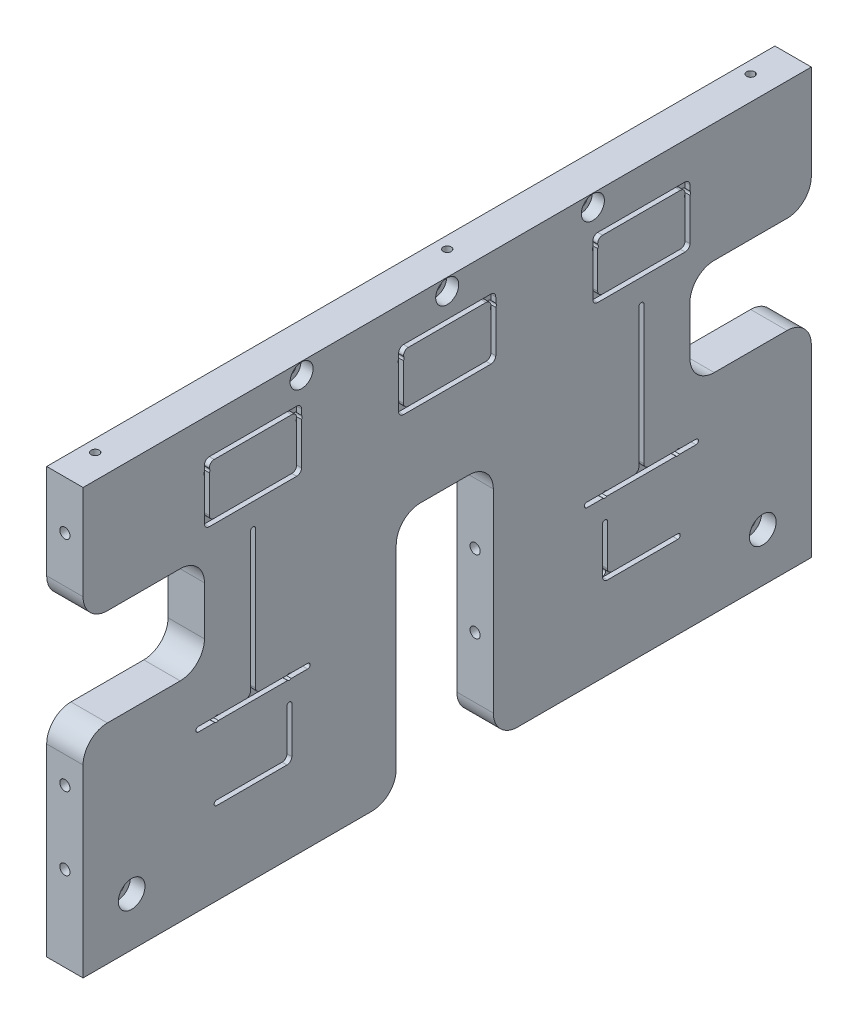
from build123d import *

# Parameters (mm, degrees)
SKETCH_2_W                                         = 300
SKETCH_2_H                                         = 175
BOSS_EXTRUDE_1_DEPTH                               = 15
SKETCH_7_W                                         = 15
SKETCH_7_H                                         = 40
CUT_EXTRUDE_1_DEPTH                                = 100
FILLET_1_R                                         = 10
SKETCH_8_W                                         = 15
SKETCH_8_H                                         = 40
CUT_EXTRUDE_2_DEPTH                                = 50
FILLET_2_R                                         = 10
SKETCH_9_R                                         = 2
CUT_EXTRUDE_3_DEPTH                                = 313.859792879
SKETCH_10_R                                        = 2
CUT_EXTRUDE_4_DEPTH                                = 313.859792879
LINEAR_PATTERN_1_COUNT                             = 2
LINEAR_PATTERN_1_PITCH                             = 30
M5_TAPPED_HOLE_1_AT_2_COUNT                        = 2
M5_TAPPED_HOLE_1_AT_2_PITCH                        = 90
M5_TAPPED_HOLE_1_AT_3_COUNT                        = 2
M5_TAPPED_HOLE_1_AT_3_PITCH                        = 120
M5_SOCKET_HEAD_CAP_SCREW_COUNTERBORE_1_D           = 5.5
M5_SOCKET_HEAD_CAP_SCREW_COUNTERBORE_1_CBORE_D     = 9.5
M5_SOCKET_HEAD_CAP_SCREW_COUNTERBORE_1_CBORE_DEPTH = 5
LINEAR_PATTERN_2_COUNT                             = 3
LINEAR_PATTERN_2_PITCH                             = 60
M6_SOCKET_HEAD_CAP_SCREW_COUNTERBORE_1_D           = 6.6
M6_SOCKET_HEAD_CAP_SCREW_COUNTERBORE_1_CBORE_D     = 11
M6_SOCKET_HEAD_CAP_SCREW_COUNTERBORE_1_CBORE_DEPTH = 6
CUT_EXTRUDE_5_DEPTH                                = 2
M5_TAPPED_HOLE_2_D                                 = 4.2
M5_TAPPED_HOLE_2_DEPTH                             = 12.4
M5_TAPPED_HOLE_2_TIP                               = 1.2618073
LINEAR_PATTERN_3_COUNT                             = 2
LINEAR_PATTERN_3_PITCH                             = 38
CUT_EXTRUDE_6_DEPTH                                = 2
LINEAR_PATTERN_4_COUNT                             = 2
LINEAR_PATTERN_4_PITCH                             = 30
LINEAR_PATTERN_5_COUNT                             = 2
LINEAR_PATTERN_5_PITCH                             = 80
LINEAR_PATTERN_6_COUNT                             = 2
LINEAR_PATTERN_6_PITCH                             = 80
CUT_EXTRUDE_7_DEPTH                                = 2
M4_TAPPED_HOLE_2_D                                 = 3.3
M4_TAPPED_HOLE_2_DEPTH                             = 10.1
M4_TAPPED_HOLE_2_TIP                               = 0.991420021
M5_TAPPED_HOLE_3_D                                 = 4.2
M5_TAPPED_HOLE_3_DEPTH                             = 12.4
M5_TAPPED_HOLE_3_TIP                               = 1.2618073


with BuildPart() as part:
    # Sketch 2 → Boss-Extrude 1 (new body)
    with BuildSketch(Plane(origin=(0, 0, 0), x_dir=(0, 0, -1), z_dir=(1, 0, 0))):
        Rectangle(SKETCH_2_W, SKETCH_2_H)
    extrude(amount=BOSS_EXTRUDE_1_DEPTH)

    # Sketch 3 → M4 Tapped Hole 1 (revolve, cut)
    with BuildSketch(Plane(origin=(5, 87.5, -135), x_dir=(0, 0, 1), z_dir=(1, 0, 0))):
        Polygon((0, 0), (0, 11.091420021), (1.65, 10.1), (1.65, 0), align=None)
    m4_tapped_hole_1 = revolve(axis=Axis((5, 93.85, -135), (0, -1, 0)), mode=Mode.SUBTRACT)

    # Mirror 1: M4 Tapped Hole 1 across plane
    add(m4_tapped_hole_1.mirror(Plane.XY), mode=Mode.SUBTRACT)

    # Sketch 7 → Cut-Extrude 1 (cut)
    with BuildSketch(Plane.XZ.offset(87.5)):
        with Locations((7.5, 1)):
            Rectangle(SKETCH_7_W, SKETCH_7_H)
    extrude(amount=-CUT_EXTRUDE_1_DEPTH, mode=Mode.SUBTRACT)

    # Fillet 1
    fillet_1_edges = [part.edges().sort_by_distance(p)[0] for p in [
        (7.5, 12.5, 21),
        (7.5, 12.5, -19),
        (7.5, -87.5, -19),
        (7.5, -87.5, 21),
    ]]
    fillet(fillet_1_edges, radius=FILLET_1_R)

    # Sketch 8 → Cut-Extrude 2 (cut)
    with BuildSketch(Plane(origin=(0, 0, -150), x_dir=(-1, 0, 0), z_dir=(0, 0, -1))):
        with Locations((-7.5, 18.5)):
            Rectangle(SKETCH_8_W, SKETCH_8_H)
    cut_extrude_2 = extrude(amount=-CUT_EXTRUDE_2_DEPTH, mode=Mode.SUBTRACT)

    # Mirror 2: Cut-Extrude 2 across plane
    add(cut_extrude_2.mirror(Plane.XY), mode=Mode.SUBTRACT)

    # Fillet 2
    fillet_2_edges = [part.edges().sort_by_distance(p)[0] for p in [
        (7.5, -1.5, -100),
        (7.5, 38.5, -100),
        (7.5, 38.5, -150),
        (7.5, -1.5, -150),
        (7.5, 38.5, 150),
        (7.5, -1.5, 150),
        (7.5, 38.5, 100),
        (7.5, -1.5, 100),
    ]]
    fillet(fillet_2_edges, radius=FILLET_2_R)

    # Sketch 9 → Cut-Extrude 3 (cut, through all)
    with BuildSketch(Plane.XY.offset(150)):
        with Locations((7.5, 67.5)):
            Circle(SKETCH_9_R)
    extrude(amount=-CUT_EXTRUDE_3_DEPTH, mode=Mode.SUBTRACT)

    # Sketch 10 → Cut-Extrude 4 (cut, through all)
    with BuildSketch(Plane.XY.offset(150)):
        with Locations((7.5, -22.5)):
            Circle(SKETCH_10_R)
    cut_extrude_4 = extrude(amount=-CUT_EXTRUDE_4_DEPTH, mode=Mode.SUBTRACT)

    # Linear Pattern 1: Cut-Extrude 4 ×2
    with Locations(*[(0, -i * LINEAR_PATTERN_1_PITCH, 0) for i in range(1, LINEAR_PATTERN_1_COUNT)]):
        add(cut_extrude_4, mode=Mode.SUBTRACT)

    # Sketch 11 → M5 Tapped Hole 1 (revolve, cut)
    with BuildSketch(Plane(origin=(7.5, 67.5, 150), x_dir=(0, -1, 0), z_dir=(1, 0, 0))):
        Polygon((0, 0), (0, 13.6618073), (2.1, 12.4), (2.1, 0), align=None)
    m5_tapped_hole_1 = revolve(axis=Axis((7.5, 67.5, 156.35), (0, 0, -1)), mode=Mode.SUBTRACT)

    # M5 Tapped Hole 1 at 2: M5 Tapped Hole 1 ×2
    with Locations(*[(0, -i * M5_TAPPED_HOLE_1_AT_2_PITCH, 0) for i in range(1, M5_TAPPED_HOLE_1_AT_2_COUNT)]):
        add(m5_tapped_hole_1, mode=Mode.SUBTRACT)

    # M5 Tapped Hole 1 at 3: M5 Tapped Hole 1 ×2
    with Locations(*[(0, -i * M5_TAPPED_HOLE_1_AT_3_PITCH, 0) for i in range(1, M5_TAPPED_HOLE_1_AT_3_COUNT)]):
        add(m5_tapped_hole_1, mode=Mode.SUBTRACT)

    # Mirror 4: M5 Tapped Hole 1 across plane
    add(m5_tapped_hole_1.mirror(Plane.XY), mode=Mode.SUBTRACT)

    # Mirror 4 copy 1 sketch → Mirror 4 copy 1 (revolve, cut)
    with BuildSketch(Plane(origin=(7.5, -22.5, -150), x_dir=(0, -1, 0), z_dir=(1, 0, 0))):
        Polygon((0, 0), (0, -13.6618073), (2.1, -12.4), (2.1, 0), align=None)
    revolve(axis=Axis((7.5, -22.5, -156.35), (0, 0, -1)), mode=Mode.SUBTRACT)

    # Mirror 4 copy 2 sketch → Mirror 4 copy 2 (revolve, cut)
    with BuildSketch(Plane(origin=(7.5, -52.5, -150), x_dir=(0, -1, 0), z_dir=(1, 0, 0))):
        Polygon((0, 0), (0, -13.6618073), (2.1, -12.4), (2.1, 0), align=None)
    revolve(axis=Axis((7.5, -52.5, -156.35), (0, 0, -1)), mode=Mode.SUBTRACT)

    # M5 Socket Head Cap Screw Counterbore 1 (through all)
    with Locations(Plane(origin=(15, 0, 0), x_dir=(0, 0, -1), z_dir=(1, 0, 0))):
        with Locations((-60, 82.5)):
            m5_socket_head_cap_screw_counterbore_1 = CounterBoreHole(M5_SOCKET_HEAD_CAP_SCREW_COUNTERBORE_1_D / 2, M5_SOCKET_HEAD_CAP_SCREW_COUNTERBORE_1_CBORE_D / 2, M5_SOCKET_HEAD_CAP_SCREW_COUNTERBORE_1_CBORE_DEPTH)

    # Linear Pattern 2: M5 Socket Head Cap Screw Counterbore 1 ×3
    with Locations(*[(0, 0, -i * LINEAR_PATTERN_2_PITCH) for i in range(1, LINEAR_PATTERN_2_COUNT)]):
        add(m5_socket_head_cap_screw_counterbore_1, mode=Mode.SUBTRACT)

    # M6 Socket Head Cap Screw Counterbore 1 (through all)
    with Locations(Plane(origin=(15, 0, 0), x_dir=(0, 0, -1), z_dir=(1, 0, 0))):
        with Locations((-130, -67.5)):
            m6_socket_head_cap_screw_counterbore_1 = CounterBoreHole(M6_SOCKET_HEAD_CAP_SCREW_COUNTERBORE_1_D / 2, M6_SOCKET_HEAD_CAP_SCREW_COUNTERBORE_1_CBORE_D / 2, M6_SOCKET_HEAD_CAP_SCREW_COUNTERBORE_1_CBORE_DEPTH)

    # Mirror 5: M6 Socket Head Cap Screw Counterbore 1 across plane
    add(m6_socket_head_cap_screw_counterbore_1.mirror(Plane.XY), mode=Mode.SUBTRACT)

    # Sketch 18 → Cut-Extrude 5 (cut)
    with BuildSketch(Plane(origin=(15, 0, 0), x_dir=(0, 0, -1), z_dir=(1, 0, 0))):
        with BuildLine():
            Line((-98, 72.5), (-62, 72.5))
            ThreePointArc((-62, 72.5), (-60.585786438, 71.914213562), (-60, 70.5))
            Line((-60, 70.5), (-60, 49.5))
            ThreePointArc((-60, 49.5), (-60.585786438, 48.085786438), (-62, 47.5))
            Line((-62, 47.5), (-98, 47.5))
            ThreePointArc((-98, 47.5), (-99.414213562, 48.085786438), (-100, 49.5))
            Line((-100, 49.5), (-100, 70.5))
            ThreePointArc((-100, 70.5), (-99.414213562, 71.914213562), (-98, 72.5))
        make_face()
        with BuildLine():
            Line((-96, 70.5), (-64, 70.5))
            ThreePointArc((-64, 70.5), (-62.585786438, 69.914213562), (-62, 68.5))
            Line((-62, 68.5), (-62, 51.5))
            ThreePointArc((-62, 51.5), (-62.585786438, 50.085786438), (-64, 49.5))
            Line((-64, 49.5), (-96, 49.5))
            ThreePointArc((-96, 49.5), (-97.414213562, 50.085786438), (-98, 51.5))
            Line((-98, 51.5), (-98, 68.5))
            ThreePointArc((-98, 68.5), (-97.414213562, 69.914213562), (-96, 70.5))
        make_face(mode=Mode.SUBTRACT)
    cut_extrude_5 = extrude(amount=-CUT_EXTRUDE_5_DEPTH, mode=Mode.SUBTRACT)

    # M5 Tapped Hole 2
    with Locations(Plane(origin=(0, 0, 21), x_dir=(-1, 0, 0), z_dir=(0, 0, -1))):
        with Locations((-7.5, -22.5), (-7.5, -52.5)):
            Hole(M5_TAPPED_HOLE_2_D / 2, depth=M5_TAPPED_HOLE_2_DEPTH)
            with Locations((0, 0, -(M5_TAPPED_HOLE_2_DEPTH + M5_TAPPED_HOLE_2_TIP / 2))):  # 118° drill point
                Cone(0, M5_TAPPED_HOLE_2_D / 2, M5_TAPPED_HOLE_2_TIP, mode=Mode.SUBTRACT)

    # Sketch 21 → M3 Tapped Hole 1 (revolve, cut)
    with BuildSketch(Plane(origin=(15, 67.5, 99), x_dir=(0, 0, -1), z_dir=(0, 1, 0))):
        Polygon((0, 0), (0, 8.251075774), (1.25, 7.5), (1.25, 0), align=None)
    m3_tapped_hole_1 = revolve(axis=Axis((21.35, 67.5, 99), (-1, 0, 0)), mode=Mode.SUBTRACT)

    # Linear Pattern 3: M3 Tapped Hole 1 ×2
    with Locations(*[(0, 0, -i * LINEAR_PATTERN_3_PITCH) for i in range(1, LINEAR_PATTERN_3_COUNT)]):
        add(m3_tapped_hole_1, mode=Mode.SUBTRACT)

    # Mirror 7: M3 Tapped Hole 1 across plane
    add(m3_tapped_hole_1.mirror(Plane.XY), mode=Mode.SUBTRACT)

    # Mirror 7 copy 1 sketch → Mirror 7 copy 1 (revolve, cut)
    with BuildSketch(Plane(origin=(15, 67.5, -61), x_dir=(0, 0, 1), z_dir=(0, 1, 0))):
        Polygon((0, 0), (0, -8.251075774), (1.25, -7.5), (1.25, 0), align=None)
    revolve(axis=Axis((21.35, 67.5, -61), (1, 0, 0)), mode=Mode.SUBTRACT)

    # Mirror 8: Cut-Extrude 5 across plane
    add(cut_extrude_5.mirror(Plane.XY), mode=Mode.SUBTRACT)

    # Sketch 23 → Cut-Extrude 6 (cut)
    with BuildSketch(Plane(origin=(15, 0, 0), x_dir=(0, 0, -1), z_dir=(1, 0, 0))):
        with BuildLine():
            Line((-102.5, -21.5), (-83, -21.5))
            ThreePointArc((-83, -21.5), (-81.585786438, -20.914213562), (-81, -19.5))
            Line((-81, -19.5), (-81, 37.5))
            ThreePointArc((-81, 37.5), (-80, 38.5), (-79, 37.5))
            Line((-79, 37.5), (-79, -19.5))
            ThreePointArc((-79, -19.5), (-78.414213562, -20.914213562), (-77, -21.5))
            Line((-77, -21.5), (-57.5, -21.5))
            ThreePointArc((-57.5, -21.5), (-56.5, -22.5), (-57.5, -23.5))
            Line((-57.5, -23.5), (-102.5, -23.5))
            ThreePointArc((-102.5, -23.5), (-103.5, -22.5), (-102.5, -21.5))
        make_face()
    cut_extrude_6 = extrude(amount=-CUT_EXTRUDE_6_DEPTH, mode=Mode.SUBTRACT)

    # Sketch 24 → M3 Tapped Hole 2 (revolve, cut)
    with BuildSketch(Plane(origin=(15, -22.5, 95), x_dir=(0, 0, -1), z_dir=(0, 1, 0))):
        Polygon((0, 0), (0, 8.251075774), (1.25, 7.5), (1.25, 0), align=None)
    m3_tapped_hole_2 = revolve(axis=Axis((21.35, -22.5, 95), (-1, 0, 0)), mode=Mode.SUBTRACT)

    # Linear Pattern 4: M3 Tapped Hole 2 ×2
    with Locations(*[(0, 0, -i * LINEAR_PATTERN_4_PITCH) for i in range(1, LINEAR_PATTERN_4_COUNT)]):
        add(m3_tapped_hole_2, mode=Mode.SUBTRACT)

    # Mirror 9: Cut-Extrude 6, M3 Tapped Hole 2 across plane
    add(cut_extrude_6.mirror(Plane.XY), mode=Mode.SUBTRACT)
    add(m3_tapped_hole_2.mirror(Plane.XY), mode=Mode.SUBTRACT)

    # Mirror 9 copy 1 sketch → Mirror 9 copy 1 (revolve, cut)
    with BuildSketch(Plane(origin=(15, -22.5, -65), x_dir=(0, 0, 1), z_dir=(0, 1, 0))):
        Polygon((0, 0), (0, -8.251075774), (1.25, -7.5), (1.25, 0), align=None)
    revolve(axis=Axis((21.35, -22.5, -65), (1, 0, 0)), mode=Mode.SUBTRACT)

    # Linear Pattern 5: Cut-Extrude 5 ×2
    with Locations(*[(0, 0, -i * LINEAR_PATTERN_5_PITCH) for i in range(1, LINEAR_PATTERN_5_COUNT)]):
        add(cut_extrude_5, mode=Mode.SUBTRACT)

    # Linear Pattern 6: M3 Tapped Hole 1 ×2
    with Locations(*[(0, 0, -i * LINEAR_PATTERN_6_PITCH) for i in range(1, LINEAR_PATTERN_6_COUNT)]):
        add(m3_tapped_hole_1, mode=Mode.SUBTRACT)

    # Linear Pattern 6 copy 1 sketch → Linear Pattern 6 copy 1 (revolve, cut)
    with BuildSketch(Plane(origin=(15, 67.5, -19), x_dir=(0, 0, -1), z_dir=(0, 1, 0))):
        Polygon((0, 0), (0, 8.251075774), (1.25, 7.5), (1.25, 0), align=None)
    revolve(axis=Axis((21.35, 67.5, -19), (-1, 0, 0)), mode=Mode.SUBTRACT)

    # Sketch 26 → Cut-Extrude 7 (cut)
    with BuildSketch(Plane(origin=(15, 0, 0), x_dir=(0, 0, -1), z_dir=(1, 0, 0))):
        with BuildLine():
            Line((-95, -51.5), (-68, -51.5))
            ThreePointArc((-68, -51.5), (-66.585786438, -50.914213562), (-66, -49.5))
            Line((-66, -49.5), (-66, -32.5))
            ThreePointArc((-66, -32.5), (-65, -31.5), (-64, -32.5))
            Line((-64, -32.5), (-64, -51.5))
            ThreePointArc((-64, -51.5), (-64.585786438, -52.914213562), (-66, -53.5))
            Line((-66, -53.5), (-95, -53.5))
            ThreePointArc((-95, -53.5), (-96, -52.5), (-95, -51.5))
        make_face()
    cut_extrude_7 = extrude(amount=-CUT_EXTRUDE_7_DEPTH, mode=Mode.SUBTRACT)

    # Mirror 10: Cut-Extrude 7 across plane
    add(cut_extrude_7.mirror(Plane.XY), mode=Mode.SUBTRACT)

    # Sketch 27 → M3 Tapped Hole 3 (revolve, cut)
    with BuildSketch(Plane(origin=(15, -52, 66), x_dir=(0, 0, -1), z_dir=(0, 1, 0))):
        Polygon((0, 0), (0, 8.251075774), (1.25, 7.5), (1.25, 0), align=None)
    m3_tapped_hole_3 = revolve(axis=Axis((21.35, -52, 66), (-1, 0, 0)), mode=Mode.SUBTRACT)

    # Mirror 11: M3 Tapped Hole 3 across plane
    add(m3_tapped_hole_3.mirror(Plane.XY), mode=Mode.SUBTRACT)

    # M4 Tapped Hole 2
    with Locations(Plane(origin=(0, 87.5, 0), x_dir=(-1, 0, 0), z_dir=(0, 1, 0))):
        with Locations((-5, -10)):
            Hole(M4_TAPPED_HOLE_2_D / 2, depth=M4_TAPPED_HOLE_2_DEPTH)
            with Locations((0, 0, -(M4_TAPPED_HOLE_2_DEPTH + M4_TAPPED_HOLE_2_TIP / 2))):  # 118° drill point
                Cone(0, M4_TAPPED_HOLE_2_D / 2, M4_TAPPED_HOLE_2_TIP, mode=Mode.SUBTRACT)

    # M5 Tapped Hole 3
    with Locations(Plane.XY.offset(-19)):
        with Locations((7.5, -52.5), (7.5, -22.5)):
            Hole(M5_TAPPED_HOLE_3_D / 2, depth=M5_TAPPED_HOLE_3_DEPTH)
            with Locations((0, 0, -(M5_TAPPED_HOLE_3_DEPTH + M5_TAPPED_HOLE_3_TIP / 2))):  # 118° drill point
                Cone(0, M5_TAPPED_HOLE_3_D / 2, M5_TAPPED_HOLE_3_TIP, mode=Mode.SUBTRACT)


solid = part.part
